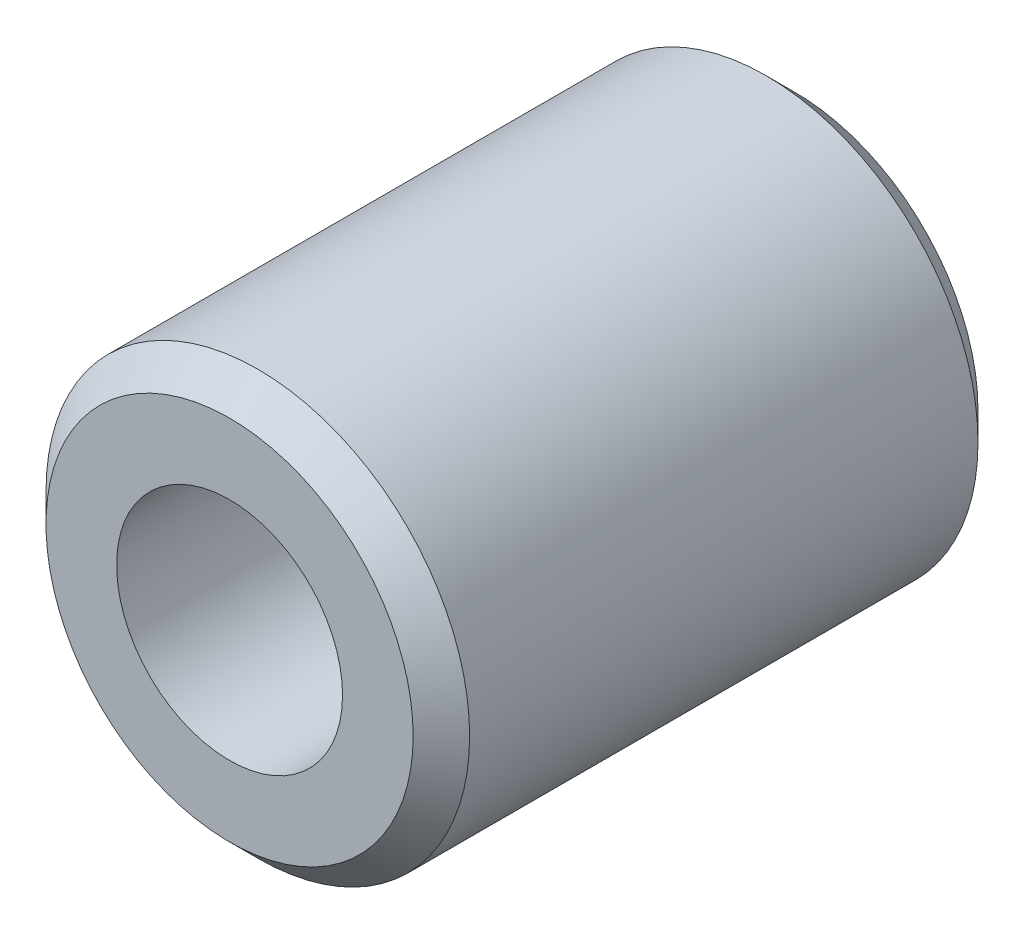
SolidWorks part; units mm, degrees
ref_plane "Front Plane" through (0, 0, 0) normal (0, 0, 1) x (1, 0, 0)
ref_plane "Top Plane" through (0, 0, 0) normal (0, 1, 0) x (1, 0, 0)
ref_plane "Right Plane" through (0, 0, 0) normal (1, 0, 0) x (0, 0, -1)
sketch "Sketch1" plane through (0, 0, 0) normal (0, 0, 1) x (1, 0, 0)
  circle A0 centre (0, 0) radius 7.5
  dimension "D1" = 15
extrude "Boss-Extrude1" add sketch "Sketch1" along normal blind 20
chamfer "Chamfer1" distance 1 angle 45 2 edges at (7.5, 0, 0) (7.5, 0, 20)
sketch "Sketch2" plane through (0, 0, 20) normal (0, 0, 1) x (1, 0, 0)
  circle A0 centre (0, 0) radius 4
  dimension "D1" = 8
extrude "Cut-Extrude1" cut sketch "Sketch2" against normal blind 20
